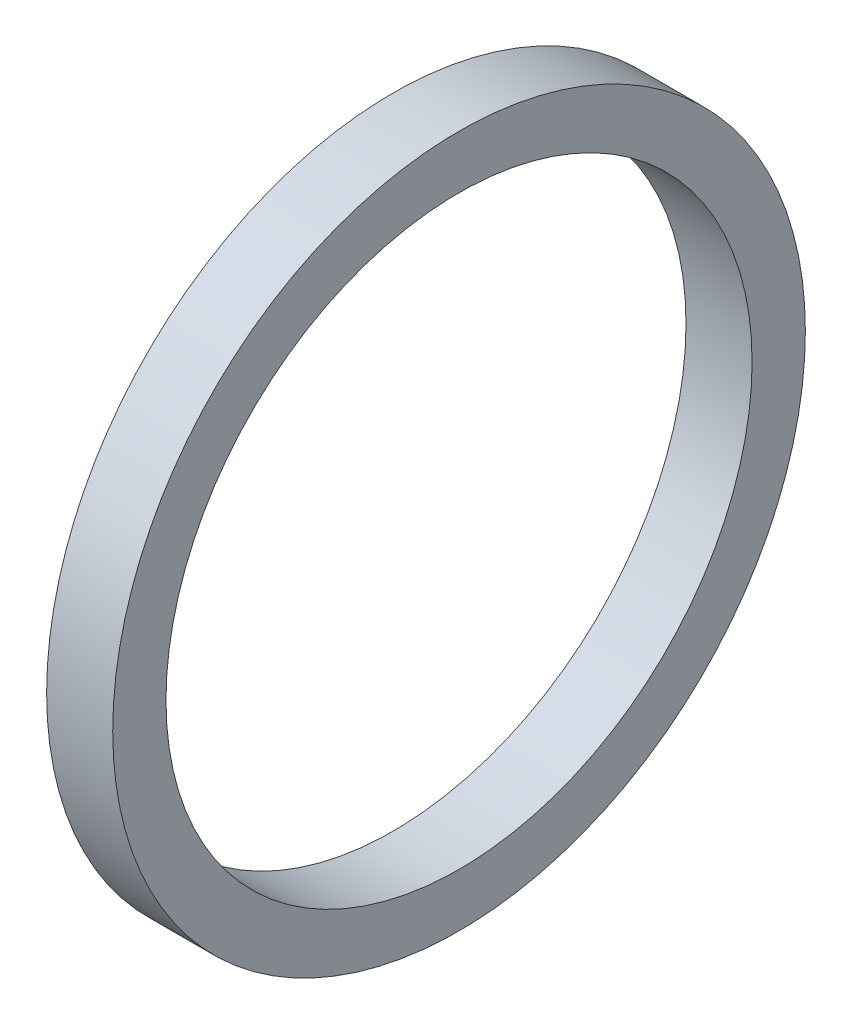
SolidWorks part; units mm, degrees
ref_plane "Front Plane" through (0, 0, 0) normal (0, 0, 1) x (1, 0, 0)
ref_plane "Top Plane" through (0, 0, 0) normal (0, 1, 0) x (1, 0, 0)
ref_plane "Right Plane" through (0, 0, 0) normal (1, 0, 0) x (0, 0, -1)
other "Configuration Table"
sketch "Sketch2" plane through (0, 0, 0) normal (1, 0, 0) x (0, 0, -1)
  circle A0 centre (0, 0) radius 27.5
  circle A1 centre (0, 0) radius 32.5
  dimension "D1" = 65
  dimension "D2" = 55
extrude "Boss-Extrude1" add sketch "Sketch2" along normal blind 6.2
